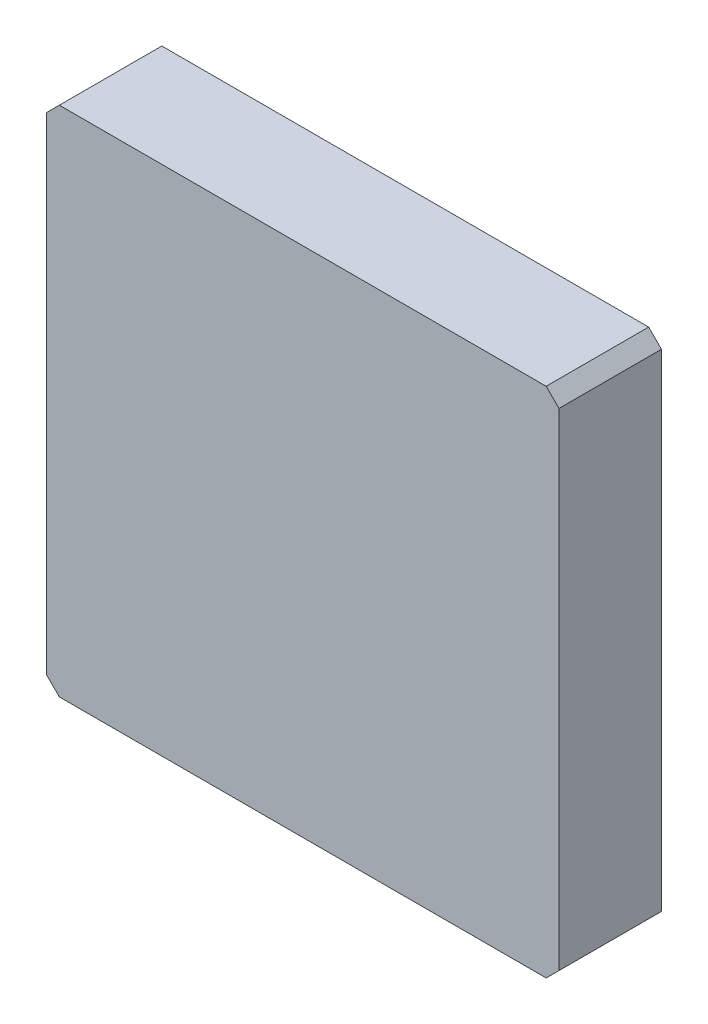
SolidWorks part; units mm, degrees
material "Q235-A"
ref_plane "Front Plane" through (0, 0, 0) normal (0, 0, 1) x (1, 0, 0)
ref_plane "Top Plane" through (0, 0, 0) normal (0, 1, 0) x (1, 0, 0)
ref_plane "Right Plane" through (0, 0, 0) normal (1, 0, 0) x (0, 0, -1)
sketch "Sketch1" plane through (0, 0, 0) normal (0, 0, 1) x (1, 0, 0)
  line L1 (-20, 20) -> (20, 20)
  line L2 (-20, 20) -> (-20, -20)
  line L3 (-20, -20) -> (20, -20)
  line L4 (20, 20) -> (20, -20)
  line L5 (-20, 20) -> (20, -20) construction
  line L6 (-20, -20) -> (20, 20) construction
  point P0 (0, 0)
  dimension "D1" = 40
extrude "Boss-Extrude1" add sketch "Sketch1" along normal blind 8
chamfer "Chamfer1" distance 1 angle 45 4 edges at (-20, -20, 4) (20, -20, 4) (20, 20, 4) (-20, 20, 4)
